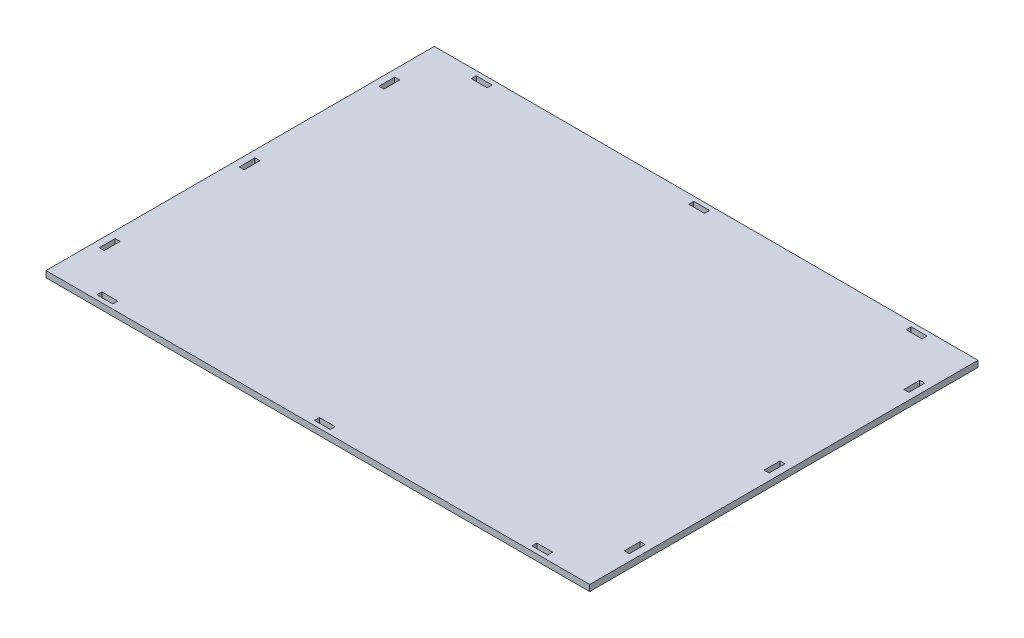
SolidWorks part; units mm, degrees
ref_plane "Front Plane" through (0, 0, 0) normal (0, 0, 1) x (1, 0, 0)
ref_plane "Top Plane" through (0, 0, 0) normal (0, 1, 0) x (1, 0, 0)
ref_plane "Right Plane" through (0, 0, 0) normal (1, 0, 0) x (0, 0, -1)
sketch "Sketch1" plane through (0, 0, 0) normal (0, 1, 0) x (1, 0, 0)
  line L1 (-175, -125) -> (175, -125)
  line L2 (-175, -125) -> (-175, 125)
  line L3 (-175, 125) -> (175, 125)
  line L4 (175, -125) -> (175, 125)
  line L5 (-175, -125) -> (175, 125) construction
  line L6 (-175, 125) -> (175, -125) construction
  point P0 (0, 0)
  dimension "D1" = 350
  dimension "D2" = 250
extrude "Boss-Extrude1" add sketch "Sketch1" along normal blind 4
sketch "Sketch2" plane through (0, 4, 0) normal (0, 1, 0) x (1, 0, 0)
  line L0 (-169, -939.6968) -> (-169, 49060.3032) construction
  line L1 (-175, 125) -> (-175, -125) construction
  line L2 (175, 125) -> (-175, 125) construction
  line L3 (-170.6, 95.1) -> (-167.4, 95.1)
  line L4 (-170.6, 95.1) -> (-170.6, 84.9)
  line L5 (-170.6, 84.9) -> (-167.4, 84.9)
  line L6 (-167.4, 95.1) -> (-167.4, 84.9)
  line L7 (-170.6, 95.1) -> (-167.4, 84.9) construction
  line L8 (-170.6, 84.9) -> (-167.4, 95.1) construction
  line L9 (-170.6, 5.1) -> (-167.4, 5.1)
  line L10 (-170.6, 5.1) -> (-170.6, -5.1)
  line L11 (-170.6, -5.1) -> (-167.4, -5.1)
  line L12 (-167.4, 5.1) -> (-167.4, -5.1)
  line L13 (-170.6, 5.1) -> (-167.4, -5.1) construction
  line L14 (-170.6, -5.1) -> (-167.4, 5.1) construction
  line L15 (-170.6, -84.9) -> (-167.4, -84.9)
  line L16 (-170.6, -84.9) -> (-170.6, -95.1)
  line L17 (-170.6, -95.1) -> (-167.4, -95.1)
  line L18 (-167.4, -84.9) -> (-167.4, -95.1)
  line L19 (-170.6, -84.9) -> (-167.4, -95.1) construction
  line L20 (-170.6, -95.1) -> (-167.4, -84.9) construction
  line L21 (-175, -125) -> (175, -125) construction
  line L22 (0, -1000) -> (0, 49000) construction
  line L23 (170.6, -95.1) -> (167.4, -84.9) construction
  line L24 (170.6, -84.9) -> (167.4, -95.1) construction
  line L25 (170.6, -5.1) -> (167.4, 5.1) construction
  line L26 (170.6, 5.1) -> (167.4, -5.1) construction
  line L27 (170.6, 84.9) -> (167.4, 95.1) construction
  line L28 (170.6, 95.1) -> (167.4, 84.9) construction
  line L29 (167.4, -84.9) -> (167.4, -95.1)
  line L30 (170.6, -95.1) -> (167.4, -95.1)
  line L31 (170.6, -84.9) -> (170.6, -95.1)
  line L32 (170.6, -84.9) -> (167.4, -84.9)
  line L33 (167.4, 5.1) -> (167.4, -5.1)
  line L34 (170.6, -5.1) -> (167.4, -5.1)
  line L35 (170.6, 5.1) -> (170.6, -5.1)
  line L36 (170.6, 5.1) -> (167.4, 5.1)
  line L37 (167.4, 95.1) -> (167.4, 84.9)
  line L38 (170.6, 84.9) -> (167.4, 84.9)
  line L39 (170.6, 95.1) -> (170.6, 84.9)
  line L40 (170.6, 95.1) -> (167.4, 95.1)
  point P4 (-169, 90)
  point P9 (-169, 0)
  point P14 (-169, -90)
  point P38 (169, -90)
  point P39 (169, 0)
  point P40 (169, 90)
  dimension "D1" = 6
  dimension "D2" = 10.2
  dimension "D3" = 3.2
  dimension "D4" = 29.9
  dimension "D5" = 10.2
  dimension "D6" = 3.2
  dimension "D7" = 10.2
  dimension "D8" = 3.2
  dimension "D9" = 29.9
extrude "Cut-Extrude1" cut sketch "Sketch2" against normal through all
sketch "Sketch3" plane through (0, 4, 0) normal (0, 1, 0) x (1, 0, 0)
  line L0 (-1011.3967, 120.5) -> (48988.6033, 120.5) construction
  line L1 (-1000, 0) -> (49000, 0) construction
  line L2 (175, 125) -> (-175, 125) construction
  line L3 (-175, 125) -> (-175, -125) construction
  line L4 (-5.1, 122.1) -> (5.1, 122.1)
  line L5 (-5.1, 122.1) -> (-5.1, 118.9)
  line L6 (-5.1, 118.9) -> (5.1, 118.9)
  line L7 (5.1, 122.1) -> (5.1, 118.9)
  line L8 (-5.1, 122.1) -> (5.1, 118.9) construction
  line L9 (-5.1, 118.9) -> (5.1, 122.1) construction
  line L10 (134.9, 122.1) -> (145.1, 122.1)
  line L11 (134.9, 122.1) -> (134.9, 118.9)
  line L12 (134.9, 118.9) -> (145.1, 118.9)
  line L13 (145.1, 122.1) -> (145.1, 118.9)
  line L14 (134.9, 122.1) -> (145.1, 118.9) construction
  line L15 (134.9, 118.9) -> (145.1, 122.1) construction
  line L16 (-145.1, 122.1) -> (-134.9, 122.1)
  line L17 (-145.1, 122.1) -> (-145.1, 118.9)
  line L18 (-145.1, 118.9) -> (-134.9, 118.9)
  line L19 (-134.9, 122.1) -> (-134.9, 118.9)
  line L20 (-145.1, 122.1) -> (-134.9, 118.9) construction
  line L21 (-145.1, 118.9) -> (-134.9, 122.1) construction
  line L22 (175, -125) -> (175, 125) construction
  line L23 (-145.1, -118.9) -> (-134.9, -122.1) construction
  line L24 (-145.1, -122.1) -> (-134.9, -118.9) construction
  line L25 (134.9, -118.9) -> (145.1, -122.1) construction
  line L26 (134.9, -122.1) -> (145.1, -118.9) construction
  line L27 (-5.1, -118.9) -> (5.1, -122.1) construction
  line L28 (-5.1, -122.1) -> (5.1, -118.9) construction
  line L29 (-134.9, -122.1) -> (-134.9, -118.9)
  line L30 (-145.1, -118.9) -> (-134.9, -118.9)
  line L31 (-145.1, -122.1) -> (-145.1, -118.9)
  line L32 (-145.1, -122.1) -> (-134.9, -122.1)
  line L33 (145.1, -122.1) -> (145.1, -118.9)
  line L34 (134.9, -118.9) -> (145.1, -118.9)
  line L35 (134.9, -122.1) -> (134.9, -118.9)
  line L36 (134.9, -122.1) -> (145.1, -122.1)
  line L37 (5.1, -122.1) -> (5.1, -118.9)
  line L38 (-5.1, -118.9) -> (5.1, -118.9)
  line L39 (-5.1, -122.1) -> (-5.1, -118.9)
  line L40 (-5.1, -122.1) -> (5.1, -122.1)
  point P7 (0, 120.5)
  point P12 (140, 120.5)
  point P17 (-140, 120.5)
  point P38 (-140, -120.5)
  point P39 (140, -120.5)
  point P40 (0, -120.5)
  dimension "D1" = 4.5
  dimension "D2" = 10.2
  dimension "D3" = 3.2
  dimension "D4" = 10.2
  dimension "D5" = 3.2
  dimension "D6" = 10.2
  dimension "D7" = 3.2
  dimension "D8" = 29.9
  dimension "D9" = 29.9
extrude "Cut-Extrude2" cut sketch "Sketch3" against normal through all
